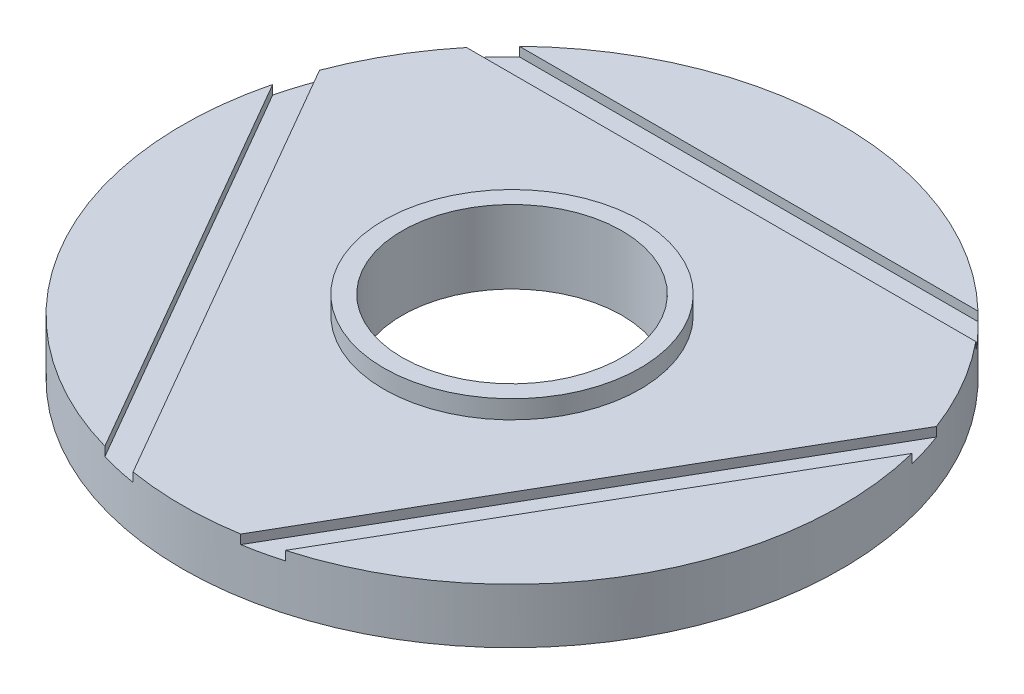
from build123d import *

# Parameters (mm, degrees)
SKETCH1_R           = 180
SKETCH1_R_2         = 60
BOSS_EXTRUDE1_DEPTH = 30
SKETCH2_R           = 70
SKETCH2_R_2         = 60
BOSS_EXTRUDE2_DEPTH = 10
SKETCH4_W           = 387.286858061
SKETCH4_H           = 15
CUT_EXTRUDE2_DEPTH  = 5
CIRPATTERN1_COUNT   = 3


with BuildPart() as part:
    # Sketch1 → Boss-Extrude1 (new body)
    with BuildSketch(Plane(origin=(0, 0, 0), x_dir=(1, 0, 0), z_dir=(0, 1, 0))):
        with Locations(Location((0, 0, 0), (0, 0, 270))):
            Circle(SKETCH1_R)
        with Locations(Location((0, 0, 0), (0, 0, 270))):
            Circle(SKETCH1_R_2, mode=Mode.SUBTRACT)
    extrude(amount=BOSS_EXTRUDE1_DEPTH)

    # Sketch2 → Boss-Extrude2 (add)
    with BuildSketch(Plane(origin=(0, 30, 0), x_dir=(1, 0, 0), z_dir=(0, 1, 0))):
        with Locations(Location((0, 0, 0), (0, 0, 270))):
            Circle(SKETCH2_R)
        with Locations(Location((0, 0, 0), (0, 0, 270))):
            Circle(SKETCH2_R_2, mode=Mode.SUBTRACT)
    extrude(amount=BOSS_EXTRUDE2_DEPTH)

    # Sketch4 → Cut-Extrude2 (cut)
    with BuildSketch(Plane(origin=(0, 30, 0), x_dir=(1, 0, 0), z_dir=(0, 1, 0))):
        with Locations((7.031744629, 121.75)):
            Rectangle(SKETCH4_W, SKETCH4_H)
    cut_extrude2 = extrude(amount=-CUT_EXTRUDE2_DEPTH, mode=Mode.SUBTRACT)

    # CirPattern1: Cut-Extrude2 ×3 about axis
    cirpattern1_axis = Axis((0, 0, 0), (0, 1, 0))
    for i in range(1, CIRPATTERN1_COUNT):
        add(cut_extrude2.rotate(cirpattern1_axis, i * 360 / CIRPATTERN1_COUNT), mode=Mode.SUBTRACT)


solid = part.part
